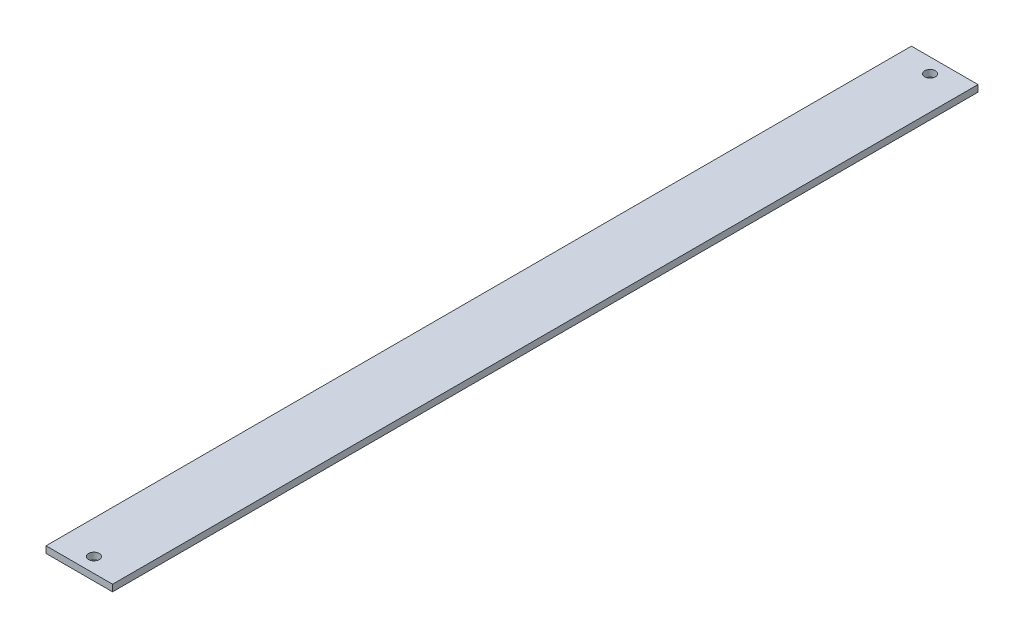
SolidWorks part; units mm, degrees
ref_plane "前视基准面" through (0, 0, 0) normal (0, 0, 1) x (1, 0, 0)
ref_plane "上视基准面" through (0, 0, 0) normal (0, 1, 0) x (1, 0, 0)
ref_plane "右视基准面" through (0, 0, 0) normal (1, 0, 0) x (0, 0, -1)
sketch "草图1" plane through (0, 0, 0) normal (0, 1, 0) x (1, 0, 0)
  line L1 (-25, 325) -> (25, 325)
  line L2 (-25, 325) -> (-25, -325)
  line L3 (-25, -325) -> (25, -325)
  line L4 (25, 325) -> (25, -325)
  line L5 (-25, 325) -> (25, -325) construction
  line L6 (-25, -325) -> (25, 325) construction
  point P0 (0, 0)
extrude "凸台-拉伸1" add sketch "草图1" along normal blind 5
sketch "草图2" plane through (0, 5, 0) normal (0, 1, 0) x (1, 0, 0)
  line L0 (0, 325) -> (0, 314) construction
  line L1 (25, 325) -> (-25, 325) construction
  line L2 (0, 0) -> (88.5798, 0) construction
  circle A0 centre (0, 314) radius 4
  circle A1 centre (0, -314) radius 4
  dimension "D2" = 8
  dimension "D1" = 11
extrude "切除-拉伸1" cut sketch "草图2" against normal through all
